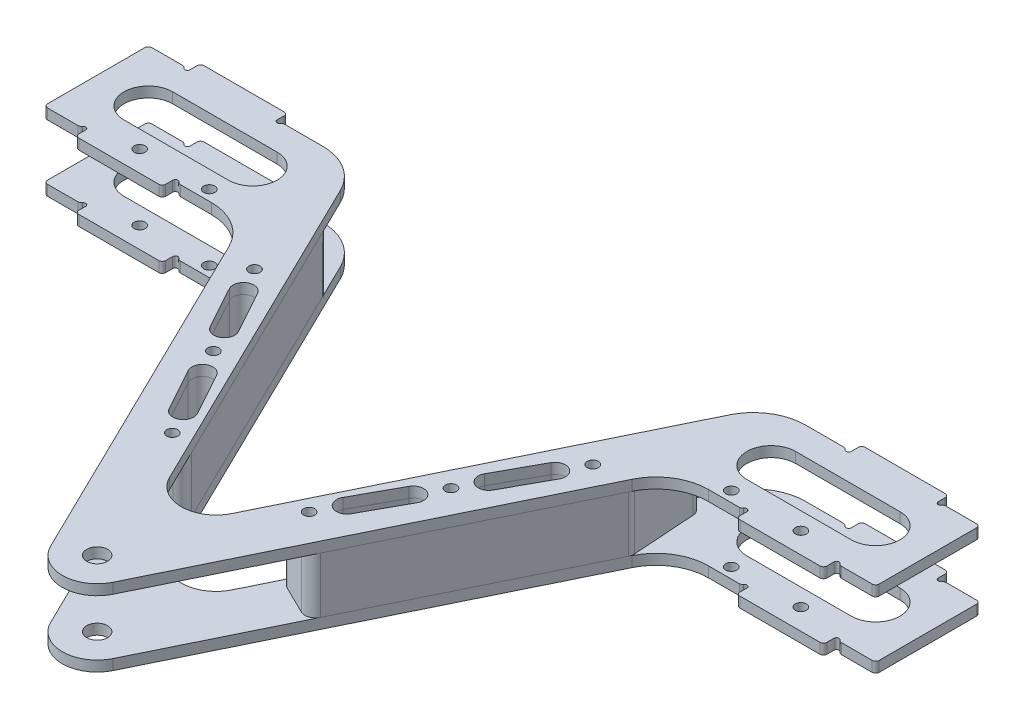
SolidWorks part; units mm, degrees
material "哈碳纤"
ref_plane "前视基准面" through (0, 0, 0) normal (0, 0, 1) x (1, 0, 0)
ref_plane "上视基准面" through (0, 0, 0) normal (0, 1, 0) x (1, 0, 0)
ref_plane "右视基准面" through (0, 0, 0) normal (1, 0, 0) x (0, 0, -1)
other "Configuration Table"
sketch "草图1" plane through (0, 0, 0) normal (0, 1, 0) x (1, 0, 0)
  line L5 (-107.5, 127) -> (-107.5, 124)
  line L6 (-107.5, 124) -> (-82.5, 124)
  line L7 (-82.5, 124) -> (-82.5, 127)
  line L8 (-82.5, 127) -> (-71.4057, 127)
  line L9 (-57.9279, 118.5839) -> (-8.9852, 18.3936)
  line L10 (0, 14.9283) -> (0, 151.0529) construction
  line L12 (-82.5, 157) -> (-82.5, 160)
  line L13 (-82.5, 160) -> (-107.5, 160)
  line L14 (-107.5, 160) -> (-107.5, 157)
  line L20 (-119.5, 157) -> (-119.5, 127)
  line L27 (107.5, 160) -> (107.5, 157)
  line L28 (82.5, 160) -> (107.5, 160)
  line L29 (82.5, 157) -> (82.5, 160)
  line L30 (57.9279, 118.5839) -> (8.9852, 18.3936)
  line L31 (82.5, 127) -> (71.4057, 127)
  line L32 (82.5, 124) -> (82.5, 127)
  line L33 (107.5, 124) -> (82.5, 124)
  line L34 (107.5, 127) -> (107.5, 124)
  line L40 (-82.5, 157) -> (-69.3666, 157)
  line L41 (-55.8888, 148.5839) -> (-8.9852, 52.5679)
  line L42 (55.8888, 148.5839) -> (8.9852, 52.5679)
  line L43 (82.5, 157) -> (69.3666, 157)
  line L44 (-107.5, 157) -> (-119.5, 157)
  line L45 (-119.5, 127) -> (-107.5, 127)
  line L46 (119.5, 127) -> (107.5, 127)
  line L47 (107.5, 157) -> (119.5, 157)
  line L48 (119.5, 157) -> (119.5, 127)
  arc A0 (-8.9852, 52.5679) -> (8.9852, 52.5679) centre (0, 56.9572) ccw
  arc A1 (-8.9852, 18.3936) -> (8.9852, 18.3936) centre (0, 22.7829) ccw
  circle A2 centre (0, 22.7829) radius 3
  circle A3 centre (0, 22.7829) radius 20 construction
  arc A4 (55.8888, 148.5839) -> (69.3666, 157) centre (69.3666, 142) cw
  arc A5 (57.9279, 118.5839) -> (71.4057, 127) centre (71.4057, 112) cw
  arc A6 (-69.3666, 157) -> (-55.8888, 148.5839) centre (-69.3666, 142) cw
  arc A7 (-71.4057, 127) -> (-57.9279, 118.5839) centre (-71.4057, 112) cw
  point P19 (60, 157)
  point P24 (0, 34.1743)
  point P28 (0, 0)
  point P41 (62.0391, 127)
  point P45 (-60, 157)
  point P48 (-62.0391, 127)
  dimension "D10" = 10
  dimension "D11" = 6
  dimension "D12" = 40
  dimension "D13" = 15
  dimension "D1" = 239
  dimension "D2" = 127
  dimension "D3" = 15
  dimension "D4" = 120
  dimension "D5" = 25
  dimension "D6" = 3
  dimension "D7" = 3
  dimension "D8" = 12
  dimension "D9" = 30
extrude "凸台-拉伸1" add sketch "草图1" along normal blind 3
sketch "草图2" plane through (0, 3, 0) normal (0, 1, 0) x (1, 0, 0)
  line L0 (-107.5, 157) -> (-119.5, 157) construction
  line L1 (-69.3666, 157) -> (-82.5, 157) construction
  line L2 (-119.5, 127) -> (-107.5, 127) construction
  line L3 (-82.5, 127) -> (-71.4057, 127) construction
  line L4 (0, 0) -> (0, 164.5887) construction
  circle A0 centre (-108.25, 157) radius 0.75
  circle A1 centre (-81.75, 157) radius 0.75
  circle A2 centre (-108.25, 127) radius 0.75
  circle A3 centre (-81.75, 127) radius 0.75
  circle A4 centre (81.75, 127) radius 0.75
  circle A5 centre (108.25, 127) radius 0.75
  circle A6 centre (81.75, 157) radius 0.75
  circle A7 centre (108.25, 157) radius 0.75
  dimension "D1" = 1.5
extrude "切除-拉伸1" cut sketch "草图2" against normal blind 3
fillet "圆角1" radius 1 20 edges at (81, 1.5, -127) (-81, 1.5, -127) (-82.5, 1.5, -124) (-107.5, 1.5, -124) (-109, 1.5, -127) (-119.5, 1.5, -127) (-109, 1.5, -157) (-107.5, 1.5, -160) (-82.5, 1.5, -160) (-81, 1.5, -157) (81, 1.5, -157) (82.5, 1.5, -160) (107.5, 1.5, -160) (109, 1.5, -157) (119.5, 1.5, -157) (119.5, 1.5, -127) (109, 1.5, -127) (107.5, 1.5, -124) (82.5, 1.5, -124) (-119.5, 1.5, -157)
sketch "草图3" plane through (0, 3, 0) normal (0, 1, 0) x (1, 0, 0)
  line L0 (-56.65, 137.3838) -> (-57.8735, 119.3838)
  line L1 (56.65, 137.3838) -> (57.8735, 119.3838)
  line L2 (-16.4208, 60.9544) -> (-24.5075, 57.004)
  line L3 (16.4208, 60.9544) -> (24.5075, 57.004)
  line L4 (0, 22.7829) -> (0, 56.9572) construction
  line L26 (71.4057, 127) -> (80.3139, 127)
  line L27 (82.5, 127) -> (82.5, 125)
  line L28 (83.5, 124) -> (106.5, 124)
  line L29 (107.5, 125) -> (107.5, 127)
  line L30 (109.6861, 127) -> (118.5, 127)
  line L31 (119.5, 128) -> (119.5, 156)
  line L32 (118.5, 157) -> (109.6861, 157)
  line L33 (107.5, 157) -> (107.5, 159)
  line L34 (106.5, 160) -> (83.5, 160)
  line L35 (82.5, 159) -> (82.5, 157)
  line L36 (80.3139, 157) -> (69.3666, 157)
  line L37 (55.8888, 148.5839) -> (8.9852, 52.5679)
  line L38 (-8.9852, 52.5679) -> (-55.8888, 148.5839)
  line L39 (-69.3666, 157) -> (-80.3139, 157)
  line L40 (-82.5, 157) -> (-82.5, 159)
  line L41 (-83.5, 160) -> (-106.5, 160)
  line L42 (-107.5, 159) -> (-107.5, 157)
  line L43 (-109.6861, 157) -> (-118.5, 157)
  line L44 (-119.5, 156) -> (-119.5, 128)
  line L45 (-118.5, 127) -> (-109.6861, 127)
  line L46 (-107.5, 127) -> (-107.5, 125)
  line L47 (-106.5, 124) -> (-83.5, 124)
  line L48 (-82.5, 125) -> (-82.5, 127)
  line L49 (-80.3139, 127) -> (-71.4057, 127)
  line L50 (-57.9279, 118.5839) -> (-8.9852, 18.3936)
  line L51 (8.9852, 18.3936) -> (57.9279, 118.5839)
  line L63 (50.9614, 138.4971) -> (15.042, 64.9667)
  line L64 (-15.042, 64.9667) -> (-50.9614, 138.4971)
  line L76 (-57.576, 117.8635) -> (-28.5199, 58.3828)
  line L77 (28.5199, 58.3828) -> (57.576, 117.8635)
  arc A34 (80.3139, 127) -> (81.1345, 127.4286) centre (80.3139, 128) ccw
  arc A35 (82.5, 127) -> (81.1345, 127.4286) centre (81.75, 127) ccw
  arc A36 (82.5, 125) -> (83.5, 124) centre (83.5, 125) ccw
  arc A37 (106.5, 124) -> (107.5, 125) centre (106.5, 125) ccw
  arc A38 (108.8655, 127.4286) -> (107.5, 127) centre (108.25, 127) ccw
  arc A39 (108.8655, 127.4286) -> (109.6861, 127) centre (109.6861, 128) ccw
  arc A40 (118.5, 127) -> (119.5, 128) centre (118.5, 128) ccw
  arc A41 (119.5, 156) -> (118.5, 157) centre (118.5, 156) ccw
  arc A42 (109.6861, 157) -> (108.8655, 156.5714) centre (109.6861, 156) ccw
  arc A43 (107.5, 157) -> (108.8655, 156.5714) centre (108.25, 157) ccw
  arc A44 (107.5, 159) -> (106.5, 160) centre (106.5, 159) ccw
  arc A45 (83.5, 160) -> (82.5, 159) centre (83.5, 159) ccw
  arc A46 (81.1345, 156.5714) -> (82.5, 157) centre (81.75, 157) ccw
  arc A47 (81.1345, 156.5714) -> (80.3139, 157) centre (80.3139, 156) ccw
  arc A48 (69.3666, 157) -> (55.8888, 148.5839) centre (69.3666, 142) ccw
  arc A49 (-8.9852, 52.5679) -> (8.9852, 52.5679) centre (0, 56.9572) ccw
  arc A50 (-55.8888, 148.5839) -> (-69.3666, 157) centre (-69.3666, 142) ccw
  arc A51 (-80.3139, 157) -> (-81.1345, 156.5714) centre (-80.3139, 156) ccw
  arc A52 (-82.5, 157) -> (-81.1345, 156.5714) centre (-81.75, 157) ccw
  arc A53 (-82.5, 159) -> (-83.5, 160) centre (-83.5, 159) ccw
  arc A54 (-106.5, 160) -> (-107.5, 159) centre (-106.5, 159) ccw
  arc A55 (-108.8655, 156.5714) -> (-107.5, 157) centre (-108.25, 157) ccw
  arc A56 (-108.8655, 156.5714) -> (-109.6861, 157) centre (-109.6861, 156) ccw
  arc A57 (-118.5, 157) -> (-119.5, 156) centre (-118.5, 156) ccw
  arc A58 (-119.5, 128) -> (-118.5, 127) centre (-118.5, 128) ccw
  arc A59 (-109.6861, 127) -> (-108.8655, 127.4286) centre (-109.6861, 128) ccw
  arc A60 (-107.5, 127) -> (-108.8655, 127.4286) centre (-108.25, 127) ccw
  arc A61 (-107.5, 125) -> (-106.5, 124) centre (-106.5, 125) ccw
  arc A62 (-83.5, 124) -> (-82.5, 125) centre (-83.5, 125) ccw
  arc A63 (-81.1345, 127.4286) -> (-82.5, 127) centre (-81.75, 127) ccw
  arc A64 (-81.1345, 127.4286) -> (-80.3139, 127) centre (-80.3139, 128) ccw
  arc A65 (-57.9279, 118.5839) -> (-71.4057, 127) centre (-71.4057, 112) ccw
  arc A66 (-8.9852, 18.3936) -> (8.9852, 18.3936) centre (0, 22.7829) ccw
  arc A67 (71.4057, 127) -> (57.9279, 118.5839) centre (71.4057, 112) ccw
  arc A138 (57.576, 117.8635) -> (57.8735, 119.3838) centre (54.8804, 119.1803) ccw
  arc A139 (56.65, 137.3838) -> (50.9614, 138.4971) centre (53.657, 137.1803) ccw
  arc A140 (24.5075, 57.004) -> (28.5199, 58.3828) centre (25.8243, 59.6996) ccw
  arc A141 (16.4208, 60.9544) -> (15.042, 64.9667) centre (17.7376, 63.65) cw
  arc A142 (-50.9614, 138.4971) -> (-56.65, 137.3838) centre (-53.657, 137.1803) ccw
  arc A143 (-57.8735, 119.3838) -> (-57.576, 117.8635) centre (-54.8804, 119.1803) ccw
  arc A144 (-24.5075, 57.004) -> (-28.5199, 58.3828) centre (-25.8243, 59.6996) cw
  arc A145 (-16.4208, 60.9544) -> (-15.042, 64.9667) centre (-17.7376, 63.65) ccw
  point P93 (-27.2031, 55.6873)
  dimension "D3" = 3
  dimension "D2" = 70
  dimension "D1" = 0
extrude "凸台-拉伸2" add sketch "草图3" along normal blind 16 separate body
ref_plane "基准面1" through (0, 11, 0) normal (0, 1, 0) x (1, 0, 0)
mirror "镜向1" about plane through (0, 11, 0) normal (0, 1, 0) of bodies 107
sketch "草图4" plane through (0, 22, 0) normal (0, 1, 0) x (1, 0, 0)
  line L0 (-8.9852, 52.5679) -> (-22.4631, 45.9841) construction
  line L1 (-57.9279, 118.5839) -> (-8.9852, 18.3936) construction
  line L2 (-13.2839, 44.2805) -> (-49.4265, 118.268) construction
  line L3 (-8.9852, 52.5679) -> (-55.8888, 148.5839) construction
  line L4 (0, 0) -> (0, 22.7829) construction
  line L5 (13.2839, 44.2805) -> (49.4265, 118.268) construction
  line L6 (8.9852, 52.5679) -> (22.4631, 45.9841) construction
  circle A0 centre (-48.6118, 116.6002) radius 1.6
  circle A1 centre (-34.1362, 90.3237) radius 1.6
  circle A2 centre (-19.6605, 64.0471) radius 1.6
  circle A3 centre (19.6605, 64.0471) radius 1.6
  circle A4 centre (34.1362, 90.3237) radius 1.6
  circle A5 centre (48.6118, 116.6002) radius 1.6
  point P6 (-15.7242, 49.276)
  dimension "D1" = 3.2
  dimension "D3" = 15
  dimension "D4" = 30
  dimension "D2" = 3
extrude "切除-拉伸2" cut sketch "草图4" against normal through all
sketch "草图5" plane through (0, 22, 0) normal (0, 1, 0) x (1, 0, 0)
  line L0 (0, 0) -> (0, 46.9572) construction
  line L2 (-118.5, 127) -> (-109.6861, 127) construction
  line L3 (-106.5, 124) -> (-83.5, 124) construction
  line L4 (-106.5, 124) -> (-83.5, 124) construction
  arc A0 (-8.9852, 52.5679) -> (8.9852, 52.5679) centre (0, 56.9572) ccw construction
  circle A1 centre (-95, 130) radius 1.6
  circle A2 centre (95, 130) radius 1.6
  circle A3 centre (-75, 130) radius 1.6
  circle A4 centre (75, 130) radius 1.6
  point P21 (-95, 124)
  dimension "D1" = 3.2
  dimension "D2" = 20
  dimension "D4" = 3
extrude "切除-拉伸3" cut sketch "草图5" against normal through all
sketch "草图6" plane through (0, 22, 0) normal (0, 1, 0) x (1, 0, 0)
  line L0 (0, 0) -> (0, 46.9572) construction
  line L1 (-44.7517, 109.5931) -> (-37.9964, 97.3307) construction
  line L2 (-42.124, 111.0407) -> (-35.3687, 98.7783)
  line L3 (-47.3793, 108.1456) -> (-40.624, 95.8832)
  line L4 (44.7517, 109.5931) -> (37.9964, 97.3307) construction
  line L5 (42.124, 111.0407) -> (35.3687, 98.7783)
  line L6 (47.3793, 108.1456) -> (40.624, 95.8832)
  line L7 (-30.276, 83.3166) -> (-23.5207, 71.0542) construction
  line L8 (-27.6484, 84.7642) -> (-20.8931, 72.5018)
  line L9 (-32.9037, 81.869) -> (-26.1484, 69.6067)
  line L10 (30.276, 83.3166) -> (23.5207, 71.0542) construction
  line L11 (27.6484, 84.7642) -> (20.8931, 72.5018)
  line L12 (32.9037, 81.869) -> (26.1484, 69.6067)
  line L13 (-104.5, 142) -> (-74.5, 142) construction
  line L14 (-104.5, 149) -> (-74.5, 149)
  line L15 (-104.5, 135) -> (-74.5, 135)
  line L16 (104.5, 142) -> (74.5, 142) construction
  line L17 (104.5, 149) -> (74.5, 149)
  line L18 (104.5, 135) -> (74.5, 135)
  line L19 (-119.5, 156) -> (-119.5, 128) construction
  line L20 (-119.5, 156) -> (-119.5, 128) construction
  line L21 (-109.6861, 157) -> (-118.5, 157) construction
  line L22 (-48.6118, 116.6002) -> (-34.1362, 90.3237) construction
  line L23 (48.6118, 116.6002) -> (34.1362, 90.3237) construction
  arc A0 (-8.9852, 52.5679) -> (8.9852, 52.5679) centre (0, 56.9572) ccw construction
  arc A1 (-42.124, 111.0407) -> (-47.3793, 108.1456) centre (-44.7517, 109.5931) ccw
  arc A2 (-40.624, 95.8832) -> (-35.3687, 98.7783) centre (-37.9964, 97.3307) ccw
  arc A3 (42.124, 111.0407) -> (47.3793, 108.1456) centre (44.7517, 109.5931) cw
  arc A4 (40.624, 95.8832) -> (35.3687, 98.7783) centre (37.9964, 97.3307) cw
  arc A5 (-27.6484, 84.7642) -> (-32.9037, 81.869) centre (-30.276, 83.3166) ccw
  arc A6 (-26.1484, 69.6067) -> (-20.8931, 72.5018) centre (-23.5207, 71.0542) ccw
  arc A7 (27.6484, 84.7642) -> (32.9037, 81.869) centre (30.276, 83.3166) cw
  arc A8 (26.1484, 69.6067) -> (20.8931, 72.5018) centre (23.5207, 71.0542) cw
  arc A9 (-104.5, 149) -> (-104.5, 135) centre (-104.5, 142) ccw
  arc A10 (-74.5, 135) -> (-74.5, 149) centre (-74.5, 142) ccw
  arc A11 (104.5, 149) -> (104.5, 135) centre (104.5, 142) cw
  arc A12 (74.5, 135) -> (74.5, 149) centre (74.5, 142) cw
  point P8 (-41.374, 103.4619)
  point P13 (-26.8984, 77.1854)
  point P16 (41.374, 103.4619)
  point P27 (-89.5, 142)
  point P30 (26.8984, 77.1854)
  point P44 (89.5, 142)
  point P50 (-119.5, 142)
  point P61 (-41.374, 103.4619)
  dimension "D1" = 8
  dimension "D2" = 30
  dimension "D3" = 30
  dimension "D4" = 6
  dimension "D5" = 14
  dimension "D6" = 30
extrude "切除-拉伸4" cut sketch "草图6" against normal through all
